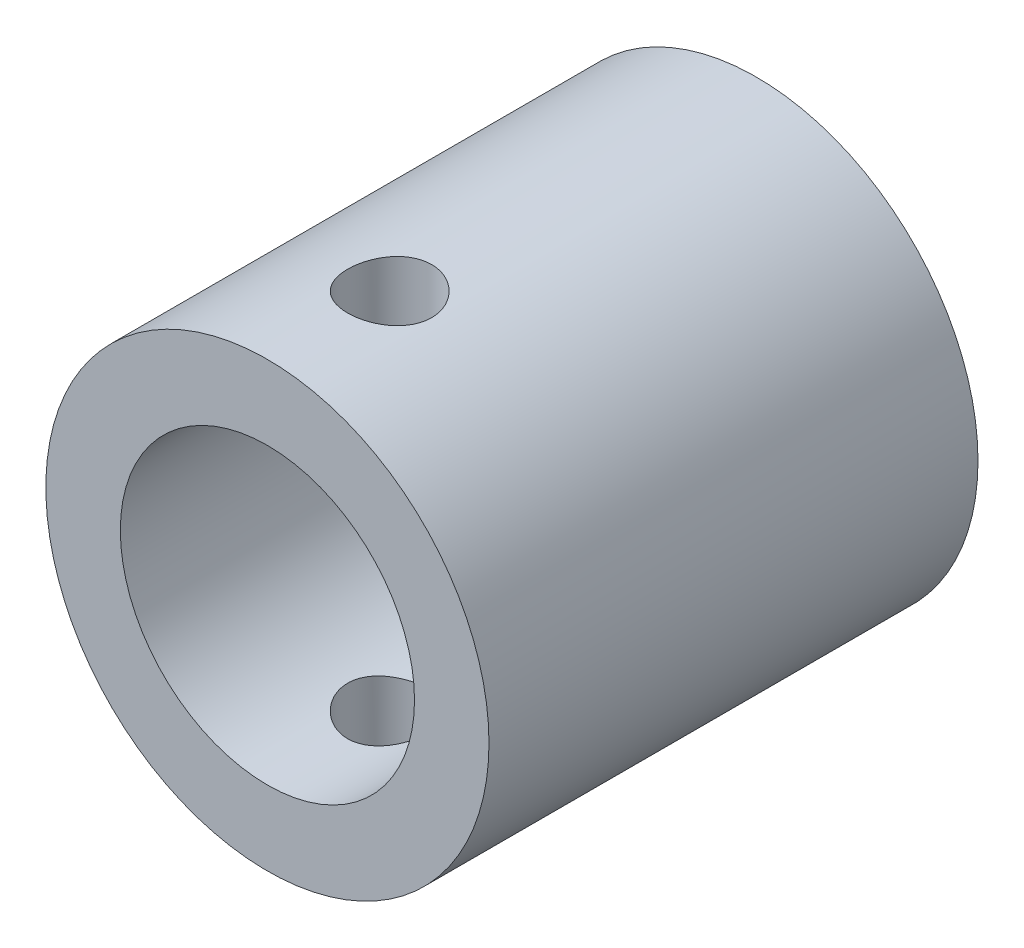
from build123d import *

# Parameters (mm, degrees)
SKETCH1_R               = 58
SKETCH1_R_2             = 24
BOSS_EXTRUDE1_DEPTH     = 128
SKETCH2_R               = 38
CUT_EXTRUDE1_DEPTH      = 102
CUT_EXTRUDE2_DEPTH      = 153.026313512
CUT_EXTRUDE2_DEPTH_BACK = 153.026313512
SKETCH3_R               = 11
SKETCH6_R               = 38.5
CUT_EXTRUDE3_DEPTH      = 68
SKETCH7_R               = 40
CUT_EXTRUDE4_DEPTH      = 4


with BuildPart() as part:
    # Sketch1 → Boss-Extrude1 (new body)
    with BuildSketch(Plane.XY):
        Circle(SKETCH1_R)
        Circle(SKETCH1_R_2, mode=Mode.SUBTRACT)
    extrude(amount=BOSS_EXTRUDE1_DEPTH)

    # Sketch2 → Cut-Extrude1 (cut)
    with BuildSketch(Plane.XY.offset(128)):
        Circle(SKETCH2_R)
    extrude(amount=-CUT_EXTRUDE1_DEPTH, mode=Mode.SUBTRACT)

    # Sketch3 → Cut-Extrude2 (cut, two sides: drawn at the far end of the back side and taken through both)
    with BuildSketch(Plane(origin=(0, 0, 0), x_dir=(1, 0, 0), z_dir=(0, 1, 0)).offset(-CUT_EXTRUDE2_DEPTH_BACK)):
        with Locations(Location((0, -96, 0), (0, 0, 270))):
            Circle(SKETCH3_R)
    extrude(amount=CUT_EXTRUDE2_DEPTH + CUT_EXTRUDE2_DEPTH_BACK, mode=Mode.SUBTRACT)

    # Sketch6 → Cut-Extrude3 (cut)
    with BuildSketch(Plane.XY.offset(128)):
        Circle(SKETCH6_R)
    extrude(amount=-CUT_EXTRUDE3_DEPTH, mode=Mode.SUBTRACT)

    # Sketch7 → Cut-Extrude4 (cut)
    with BuildSketch(Plane.XY.offset(60)):
        Circle(SKETCH7_R)
    extrude(amount=CUT_EXTRUDE4_DEPTH, mode=Mode.SUBTRACT)


solid = part.part
